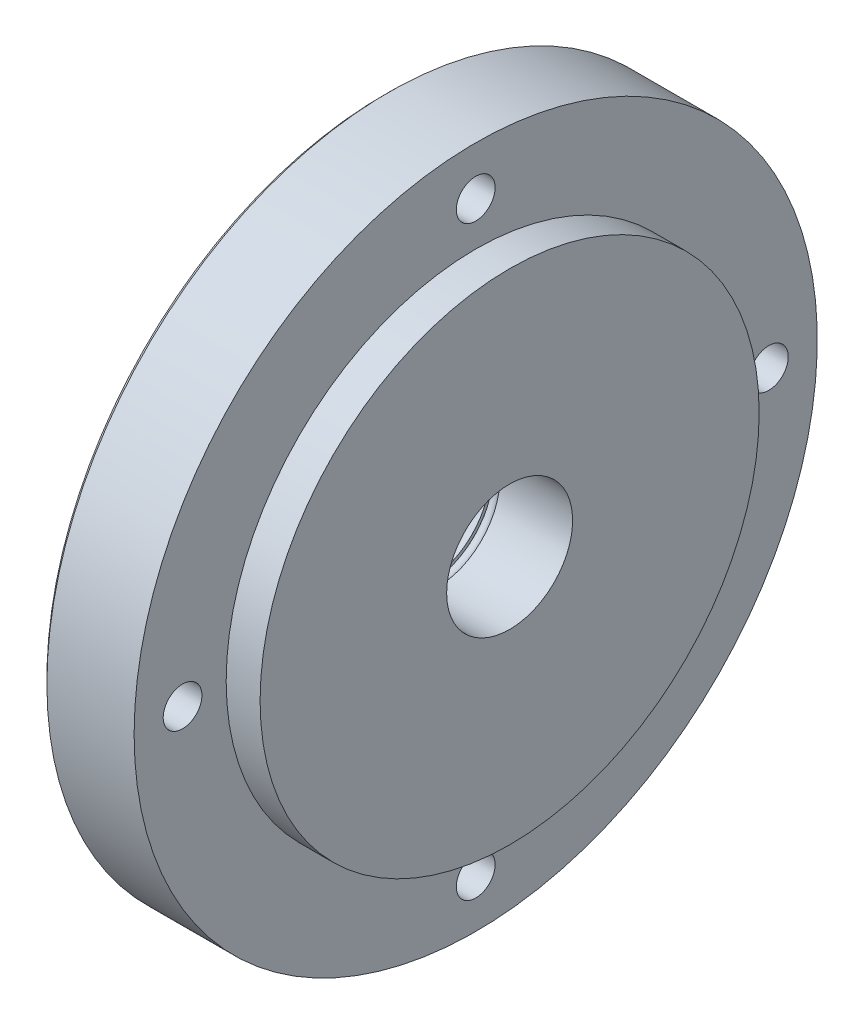
SolidWorks part; units mm, degrees
ref_plane "Front Plane" through (0, 0, 0) normal (0, 0, 1) x (1, 0, 0)
ref_plane "Top Plane" through (0, 0, 0) normal (0, 1, 0) x (1, 0, 0)
ref_plane "Right Plane" through (0, 0, 0) normal (1, 0, 0) x (0, 0, -1)
sketch "Sketch1" plane through (0, 0, 0) normal (0, 0, 1) x (1, 0, 0)
  line L0 (-70.8449, 0) -> (80.0856, 0) construction
  line L1 (-47.5722, 13) -> (-47.5722, 31)
  line L2 (-47.5722, 31) -> (-41.5722, 31)
  line L3 (-41.5722, 31) -> (-41.5722, 70.5)
  line L4 (-41.5722, 70.5) -> (-22.5722, 70.5)
  line L5 (-22.5722, 70.5) -> (-22.5722, 51.5)
  line L6 (-22.5722, 51.5) -> (-15.5722, 51.5)
  line L7 (-15.5722, 51.5) -> (-15.5722, 13)
  line L8 (-47.5722, 13) -> (-32.5722, 13)
  line L9 (-30.5722, 13) -> (-30.5722, 15)
  line L10 (-30.5722, 15) -> (-32.5722, 15)
  line L11 (-32.5722, 15) -> (-32.5722, 13)
  line L12 (-30.5722, 13) -> (-15.5722, 13)
  dimension "D1" = 32
  dimension "D2" = 13
  dimension "D3" = 18
  dimension "D4" = 26
  dimension "D5" = 19
  dimension "D6" = 51.5
  dimension "D7" = 2
  dimension "D8" = 2
  dimension "D9" = 70.5
  dimension "D10" = 15
revolve "Revolve1" add sketch "Sketch1" angle 360 about L0
chamfer "Chamfer1" distance 0.5 angle 45 1 edges at (-47.5722, 0, 31)
chamfer "Chamfer2" distance 1 angle 45 1 edges at (-41.5722, 0, 70.5)
sketch "Sketch2" plane through (-41.5722, 0, 0) normal (-1, 0, 0) x (0, 0, 1)
  circle A1 centre (0, -60.5) radius 4
  circle A2 centre (-60.5, 0) radius 4
  circle A3 centre (0, 60.5) radius 4
  circle A4 centre (60.5, 0) radius 4
  point P14 (0, 0)
  dimension "D2" = 8
  dimension "D3" = 4
extrude "Cut-Extrude2" cut sketch "Sketch2" against normal blind 61
sketch "Sketch6" plane through (-41.5722, 0, 0) normal (-1, 0, 0) x (0, 0, 1)
  circle A0 centre (0, -60.5) radius 7
  circle A1 centre (-60.5, 0) radius 7
  circle A2 centre (60.5, 0) radius 7
  circle A3 centre (0, 60.5) radius 7
  dimension "D1" = 14
  dimension "D2" = 14
  dimension "D3" = 14
  dimension "D4" = 14
extrude "Cut-Extrude3" cut sketch "Sketch6" against normal blind 6
sketch "Sketch8" plane through (0, 0, 0) normal (0, 0, 1) x (1, 0, 0)
  line L0 (-55.0437, 0) -> (3.0276, 0) construction
  circle A0 centre (-31.5722, 14) radius 1
revolve "Revolve3" add sketch "Sketch8" angle 360 about L0
sketch "Sketch9" plane through (-41.5722, 0, 0) normal (-1, 0, 0) x (0, 0, 1)
  circle A0 centre (42.78, -42.78) radius 4
  circle A1 centre (42.78, 42.78) radius 4
  circle A2 centre (-42.78, -42.78) radius 4
  circle A3 centre (-42.78, 42.78) radius 4
  point P13 (0, 0)
  dimension "D2" = 8
  dimension "D1" = 4
extrude "Cut-Extrude4" cut sketch "Sketch9" against normal blind 10
